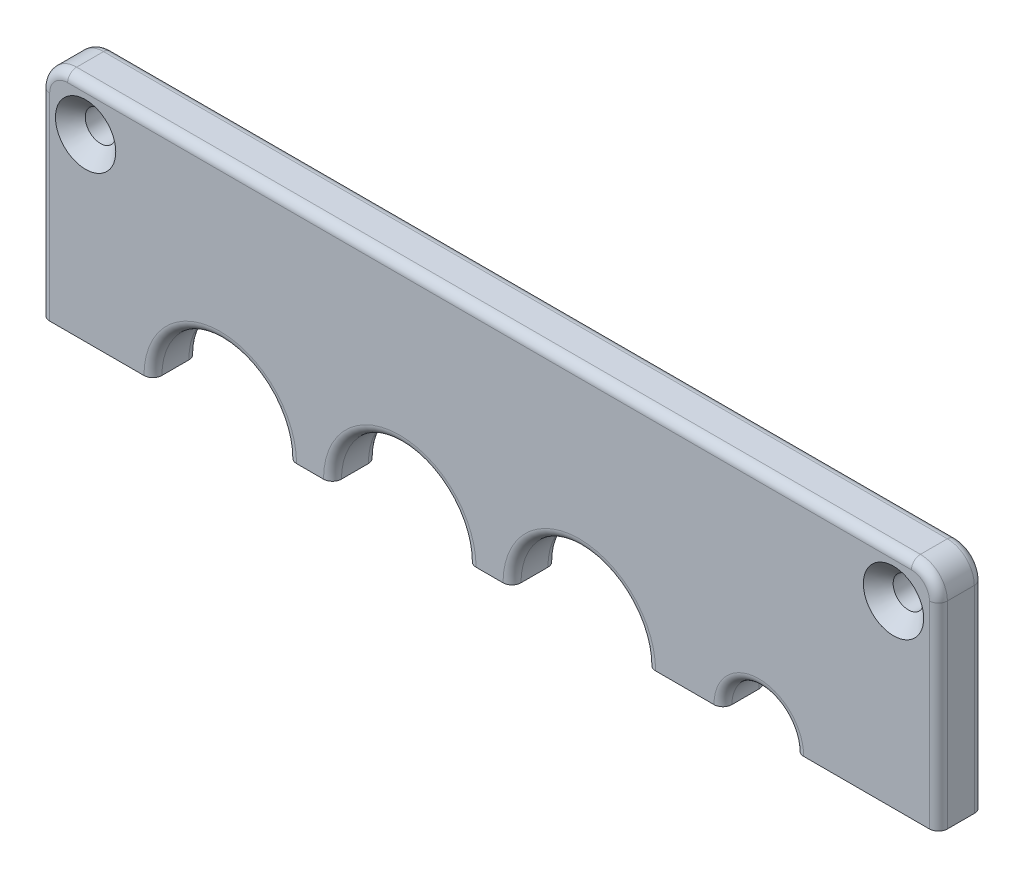
from build123d import *

# Parameters (mm, degrees)
SKETCH_1_W                   = 100
SKETCH_1_H                   = 25
EXTRUDE_1_DEPTH              = 5
SKETCH_2_R                   = 7.5
SKETCH_2_R_2                 = 4
CUT_EXTRUDE_1_DEPTH          = 104.198837203
HOLE_WIZARD_M3_1_D           = 3.4
HOLE_WIZARD_M3_1_CSINK_D     = 6.72
HOLE_WIZARD_M3_1_CSINK_ANGLE = 90
FILLET_1_R                   = 3
FILLET_2_R                   = 1


with BuildPart() as part:
    # 草图1 → 凸台-拉伸1 (new body)
    with BuildSketch(Plane.XY):
        with Locations((50, 12.5)):
            Rectangle(SKETCH_1_W, SKETCH_1_H)
    extrude(amount=EXTRUDE_1_DEPTH)

    # 草图2 → 切除-拉伸1 (cut, through all)
    with BuildSketch(Plane.XY.offset(5)):
        with Locations((20, 0)):
            Circle(SKETCH_2_R)
        with Locations((40, 0)):
            Circle(SKETCH_2_R)
        with Locations((60, 0)):
            Circle(SKETCH_2_R)
        with Locations((80, 0)):
            Circle(SKETCH_2_R_2)
    extrude(amount=-CUT_EXTRUDE_1_DEPTH, mode=Mode.SUBTRACT)

    # M3 六角凹锥坑螺钉的锥形沉头孔1 (through all)
    with Locations(Plane.XY.offset(5)):
        with Locations((5, 20), (95, 20)):
            CounterSinkHole(HOLE_WIZARD_M3_1_D / 2, HOLE_WIZARD_M3_1_CSINK_D / 2, counter_sink_angle=HOLE_WIZARD_M3_1_CSINK_ANGLE)

    # 圆角1
    fillet_1_edges = [part.edges().sort_by_distance(p)[0] for p in [
        (0, 25, 2.5),
        (100, 25, 2.5),
    ]]
    fillet(fillet_1_edges, radius=FILLET_1_R)

    # 圆角2
    fillet_2_edges = [part.edges().sort_by_distance(p)[0] for p in [
        (100, 11, 5),
        (20, 7.5, 5),
        (20, 7.5, 0),
        (40, 7.5, 5),
        (40, 7.5, 0),
        (60, 7.5, 5),
        (60, 7.5, 0),
        (80, 4, 5),
        (80, 4, 0),
        (100, 11, 0),
        (50, 25, 0),
        (50, 25, 5),
        (0, 11, 0),
        (0.878679656, 24.121320344, 0),
        (99.121320344, 24.121320344, 0),
        (0, 11, 5),
        (0.878679656, 24.121320344, 5),
        (99.121320344, 24.121320344, 5),
    ]]
    fillet(fillet_2_edges, radius=FILLET_2_R)


solid = part.part
